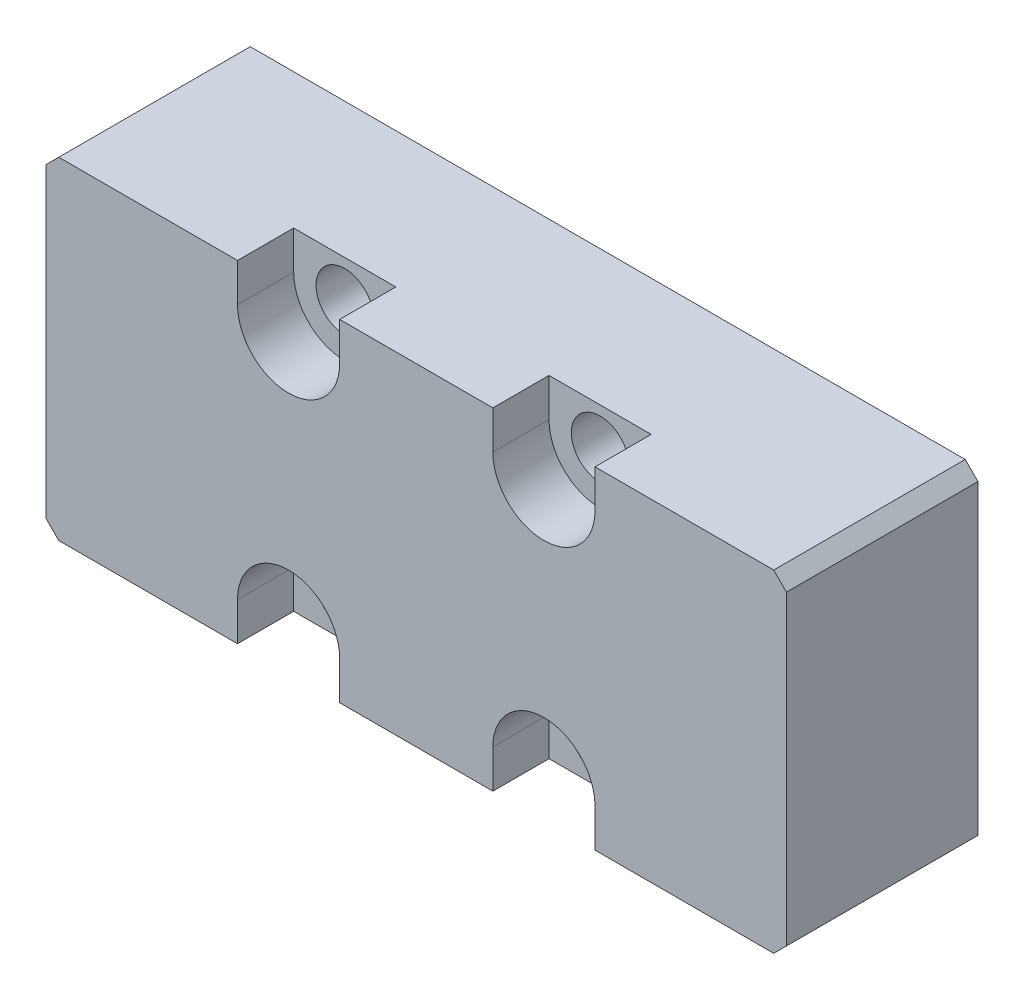
SolidWorks part; units mm, degrees
material "BPOM "
ref_plane "Front Plane" through (0, 0, 0) normal (0, 0, 1) x (1, 0, 0)
ref_plane "Top Plane" through (0, 0, 0) normal (0, 1, 0) x (1, 0, 0)
ref_plane "Right Plane" through (0, 0, 0) normal (1, 0, 0) x (0, 0, -1)
sketch "Sketch1" plane through (0, 0, 0) normal (0, 0, 1) x (1, 0, 0)
  line L1 (-29, 13) -> (29, 13)
  line L2 (-29, 13) -> (-29, -13)
  line L3 (-29, -13) -> (29, -13)
  line L4 (29, 13) -> (29, -13)
  line L5 (-29, 13) -> (29, -13) construction
  line L6 (-29, -13) -> (29, 13) construction
  point P0 (0, 0)
  dimension "D1" = 58
  dimension "D2" = 26
extrude "Boss-Extrude1" add sketch "Sketch1" along normal mid plane 15
hole_wizard "CBORE for M4 Hex Socket Head Cap Screw1" positions "Sketch4" profile "Sketch5" counterbore size "M4" standard "ISO" end condition through all
sketch "Sketch4" plane through (0, 0, 7.5) normal (0, 0, 1) x (1, 0, 0)
  point P0 (-10, 10)
  point P3 (-10, -10)
  point P6 (10, -10)
  point P9 (10, 10)
sketch "Sketch5" plane through (-10, 10, 7.5) normal (1, 0, 0) x (0, -1, 0)
  line L0 (0, 0) -> (0, 15)
  line L1 (0, 15) -> (2.25, 15)
  line L3 (2.25, 15) -> (2.25, 4.4)
  line L4 (2.25, 4.4) -> (4, 4.4)
  line L5 (4, 4.4) -> (4, 0)
  line L7 (4, 0) -> (0, 0)
  line L11 (0, -6.35) -> (0, 107.95) construction
  dimension "通孔孔直径" = 4.5
  dimension "通孔孔深度" = 15
  dimension "柱形沉头孔直径" = 8
  dimension "柱形沉头孔深度" = 4.4
sketch "Sketch6" plane through (0, 0, 7.5) normal (0, 0, 1) x (1, 0, 0)
  line L0 (7.3542, 13) -> (-7.3542, 13) construction
  line L1 (-14, 13) -> (-6, 13)
  line L2 (-14, 13) -> (-14, 10)
  line L3 (-14, 10) -> (-6, 10)
  line L4 (-6, 13) -> (-6, 10)
  line L5 (-14, 13) -> (-6, 10) construction
  line L6 (-14, 10) -> (-6, 13) construction
  line L7 (6, 13) -> (14, 13)
  line L8 (6, 13) -> (6, 10)
  line L9 (6, 10) -> (14, 10)
  line L10 (14, 13) -> (14, 10)
  line L11 (6, 13) -> (14, 10) construction
  line L12 (6, 10) -> (14, 13) construction
  arc A0 (-12.6458, 13) -> (-7.3542, 13) centre (-10, 10) ccw construction
  arc A1 (7.3542, 13) -> (12.6458, 13) centre (10, 10) ccw construction
  point P0 (-10, 11.5)
  point P5 (10, 11.5)
extrude "Cut-Extrude1" cut sketch "Sketch6" against normal up to surface (4.4 mm away) up to face at (12.25, 10, 3.1)
mirror "Mirror1" about plane through (0, 0, 0) normal (0, 1, 0) of "Cut-Extrude1"
hole_wizard "Blind Pin Hole1 (size mm)" positions "Sketch7" profile "Sketch8" hole size "Ø5.0" standard "ISO"
sketch "Sketch7" plane through (0, 0, -7.5) normal (0, 0, -1) x (-1, 0, 0)
  point P2 (-12.5, 0)
  point P5 (12.5, 0)
sketch "Sketch8" plane through (12.5, 0, -7.5) normal (1, 0, 0) x (0, 1, 0)
  line L0 (0, 0) -> (0, 3.5022)
  line L1 (0, 3.5022) -> (2.5, 2)
  line L2 (2.5, 2) -> (2.5, 0)
  line L5 (2.5, 0) -> (0, 0)
  line L10 (0, 3.5022) -> (-2.5, 2) construction
  line L11 (0, -6.35) -> (0, 107.95) construction
  dimension "孔直径" = 5
  dimension "孔深度" = 2
  dimension "导头角度" = 118
chamfer "Chamfer1" distance 1 angle 45 4 edges at (29, -13, 0) (29, 13, 0) (-29, 13, 0) (-29, -13, 0)
